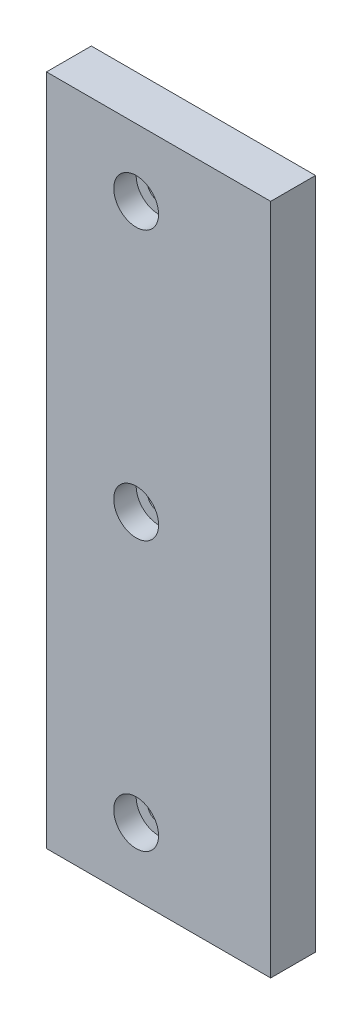
SolidWorks part; units mm, degrees
material "PA Type 6 Nylon"
ref_plane "Front Plane" through (0, 0, 0) normal (0, 0, 1) x (1, 0, 0)
ref_plane "Top Plane" through (0, 0, 0) normal (0, 1, 0) x (1, 0, 0)
ref_plane "Right Plane" through (0, 0, 0) normal (1, 0, 0) x (0, 0, -1)
sketch "Sketch1" plane through (0, 0, 0) normal (0, 0, 1) x (1, 0, 0)
  line L1 (25, -75) -> (-25, -75)
  line L2 (25, -75) -> (25, 75)
  line L3 (25, 75) -> (-25, 75)
  line L4 (-25, -75) -> (-25, 75)
  line L5 (25, -75) -> (-25, 75) construction
  line L6 (25, 75) -> (-25, -75) construction
  point P0 (0, 0)
  dimension "D1" = 150
  dimension "D2" = 50
extrude "Boss-Extrude1" add sketch "Sketch1" along normal mid plane 10
hole_wizard "Hole1" positions "Sketch2" profile "Sketch3" legacy end condition up to next
sketch "Sketch2" plane through (0, 0, 5) normal (0, 0, 1) x (1, 0, 0)
  line L0 (0, 75) -> (0, 0) construction
  line L1 (25, 75) -> (-25, 75) construction
  line L2 (0, 0) -> (-25, 0) construction
  line L3 (-25, 75) -> (-25, -75) construction
  line L4 (25, -75) -> (25, 75) construction
  point P0 (-5, 60)
  point P15 (-5, -60)
  point P16 (-5, 0)
  dimension "D1" = 30
  dimension "D2" = 120
sketch "Sketch3" plane through (-5, 60, 5) normal (1, 0, 0) x (0, -1, 0)
  line L0 (0, 0) -> (0, 10)
  line L1 (0, 10) -> (2.5, 10)
  line L2 (2.5, 10) -> (2.5, 5)
  line L3 (2.5, 5) -> (5, 5)
  line L4 (5, 5) -> (5, 0)
  line L5 (5, 0) -> (0, 0)
  line L6 (0, 110) -> (0, -10) construction
  dimension "直径" = 5
  dimension "深度" = 10
  dimension "柱坑直径" = 10
  dimension "柱坑深度" = 5
chamfer "Chamfer1" [suppressed] distance 10 angle 45
